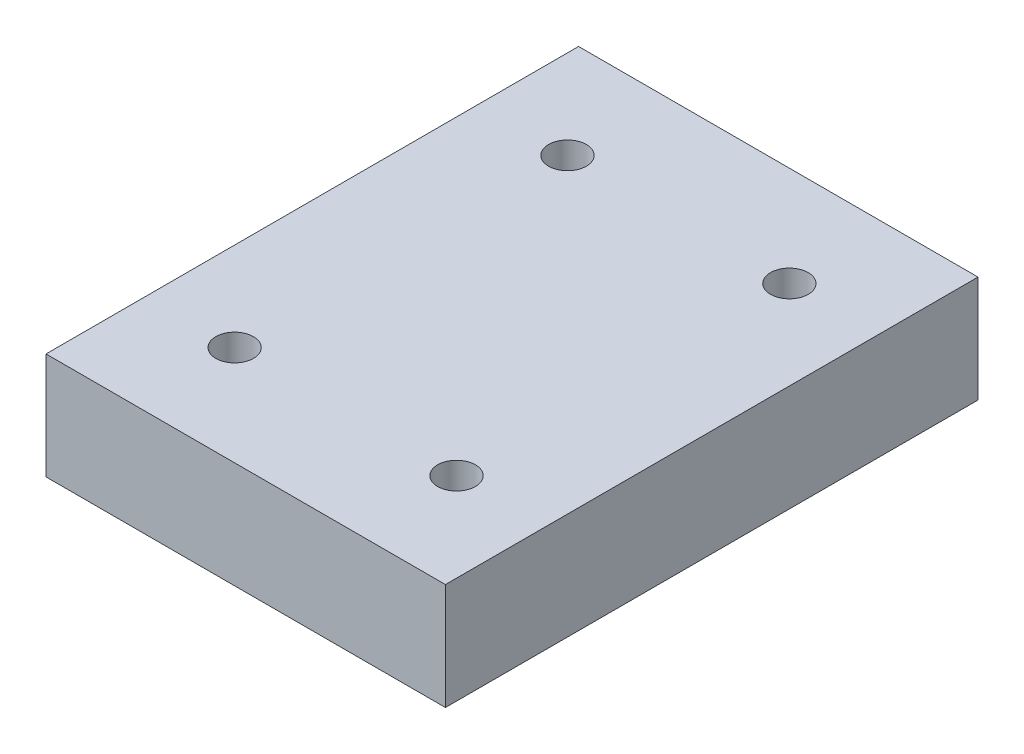
from build123d import *

# Parameters (mm, degrees)
SKETCH_1_W          = 90
SKETCH_1_H          = 120
EXTRUDE_1_DEPTH     = 24
HOLE_WIZARD_M10_1_D = 8.5


with BuildPart() as part:
    # 草图1 → 凸台-拉伸1 (new body)
    with BuildSketch(Plane(origin=(0, 0, 0), x_dir=(1, 0, 0), z_dir=(0, 1, 0))):
        Rectangle(SKETCH_1_W, SKETCH_1_H)
    extrude(amount=EXTRUDE_1_DEPTH)

    # M10 螺纹孔1 (through all)
    with Locations(Plane(origin=(0, 24, 0), x_dir=(1, 0, 0), z_dir=(0, 1, 0))):
        with Locations((-25, -37.5), (-25, 37.5), (25, 37.5), (25, -37.5)):
            Hole(HOLE_WIZARD_M10_1_D / 2)


solid = part.part
